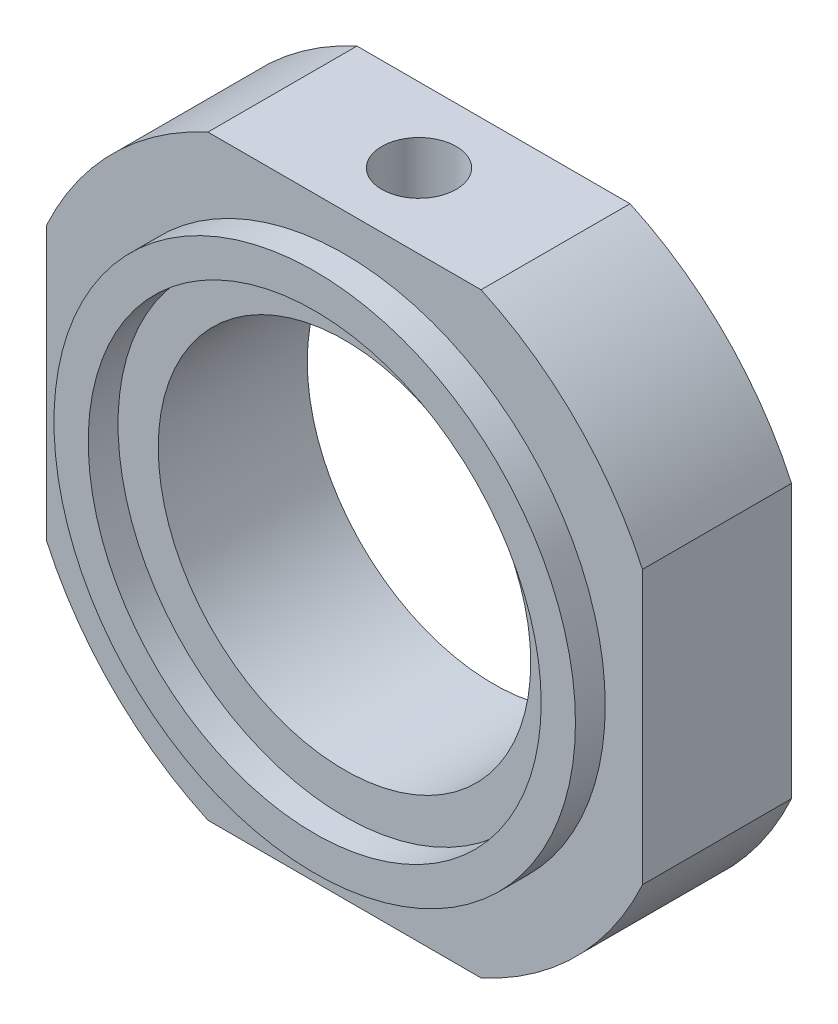
from build123d import *

# Parameters (mm, degrees)
SKETCH7_R              = 11
BOSS_EXTRUDE1_DEPTH    = 2.5
SKETCH8_R              = 8.75
SKETCH8_R_2            = 7.6
BOSS_EXTRUDE2_DEPTH    = 1
M14X1_5_TAPPED_HOLE1_D = 12.5
SKETCH13_OUTSIDE_W     = 30.338
SKETCH13_OUTSIDE_H     = 30.338
SKETCH13_OUTSIDE_W_2   = 20
SKETCH13_OUTSIDE_H_2   = 20
CUT_EXTRUDE1_DEPTH     = 17.673332001
M3_TAPPED_HOLE3_REACH  = 24.633
M3_TAPPED_HOLE3_BORE_R = 1.25


with BuildPart() as part:
    # Sketch7 → Boss-Extrude1 (new, symmetric)
    with BuildSketch(Plane.XY):
        Circle(SKETCH7_R)
    extrude(amount=BOSS_EXTRUDE1_DEPTH, both=True)

    # Sketch8 → Boss-Extrude2 (add)
    with BuildSketch(Plane.XY.offset(2.5)):
        Circle(SKETCH8_R)
        Circle(SKETCH8_R_2, mode=Mode.SUBTRACT)
    extrude(amount=BOSS_EXTRUDE2_DEPTH)

    # M14x1.5 Tapped Hole1 (through all)
    with Locations(Plane(origin=(0, 0, -2.5), x_dir=(-1, 0, 0), z_dir=(0, 0, -1))):
        with Locations((0, 0)):
            Hole(M14X1_5_TAPPED_HOLE1_D / 2)

    # Sketch13 outside → Cut-Extrude1 (cut, through all)
    with BuildSketch(Plane(origin=(0, 0, -2.5), x_dir=(-1, 0, 0), z_dir=(0, 0, -1))):
        Rectangle(SKETCH13_OUTSIDE_W, SKETCH13_OUTSIDE_H)
        Rectangle(SKETCH13_OUTSIDE_W_2, SKETCH13_OUTSIDE_H_2, mode=Mode.SUBTRACT)
    extrude(amount=-CUT_EXTRUDE1_DEPTH, mode=Mode.SUBTRACT)

    # M3 Tapped Hole3 bore → M3 Tapped Hole3 (cut, up to next)
    with BuildSketch(Plane(origin=(0, 10, 0), x_dir=(1, 0, 0), z_dir=(0, 1, 0)), mode=Mode.PRIVATE) as m3_tapped_hole3_sk1:
        Circle(M3_TAPPED_HOLE3_BORE_R)
    m3_tapped_hole3_tool1 = extrude(m3_tapped_hole3_sk1.sketch, amount=-M3_TAPPED_HOLE3_REACH, mode=Mode.PRIVATE) & part.part
    add(m3_tapped_hole3_tool1.solids().sort_by_distance((0, 10, 0))[0], mode=Mode.SUBTRACT)


solid = part.part
